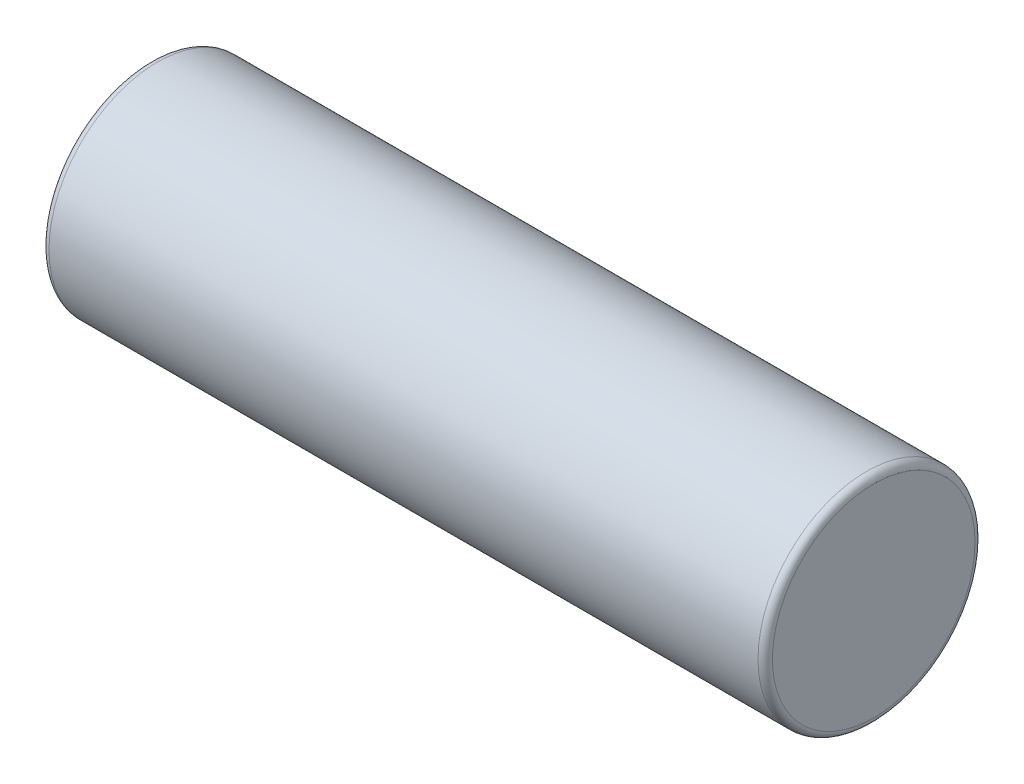
from build123d import *

# Parameters (mm, degrees)
SKETCH1_R           = 30
BOSS_EXTRUDE1_DEPTH = 200
FILLET1_R           = 2


with BuildPart() as part:
    # Sketch1 → Boss-Extrude1 (new body)
    with BuildSketch(Plane(origin=(0, 0, 0), x_dir=(0, 0, -1), z_dir=(1, 0, 0))):
        Circle(SKETCH1_R)
    extrude(amount=BOSS_EXTRUDE1_DEPTH)

    # Fillet1
    fillet1_edges = [part.edges().sort_by_distance(p)[0] for p in [
        (0, 0, 30),
        (200, 0, 30),
    ]]
    fillet(fillet1_edges, radius=FILLET1_R)


solid = part.part
